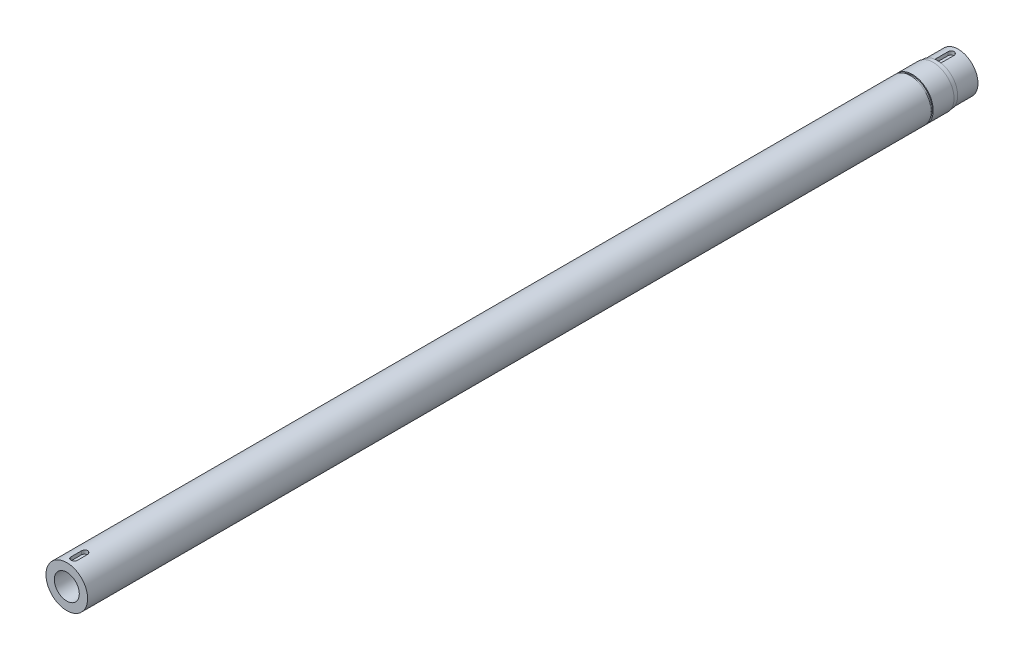
from build123d import *

# Parameters (mm, degrees)
SKETCH1_R           = 9.5
SKETCH1_R_2         = 6
BOSS_EXTRUDE1_DEPTH = 10
CUT_EXTRUDE1_DEPTH  = 1.8
CUT_EXTRUDE2_START  = 1.8
CUT_EXTRUDE2_DEPTH  = 1.8
SKETCH4_R           = 9.75
SKETCH4_R_2         = 6
BOSS_EXTRUDE2_DEPTH = 2
SKETCH5_R           = 10
BOSS_EXTRUDE3_DEPTH = 10
SKETCH6_R           = 6
CUT_EXTRUDE3_DEPTH  = 27.153393745
SKETCH7_R           = 9.5
SKETCH7_R_2         = 6
BOSS_EXTRUDE4_DEPTH = 1
SKETCH8_R           = 10
SKETCH8_R_2         = 6
BOSS_EXTRUDE5_DEPTH = 6
SKETCH9_R           = 10
SKETCH9_R_2         = 6
BOSS_EXTRUDE6_DEPTH = 150
SKETCH10_R          = 10
SKETCH10_R_2        = 6
BOSS_EXTRUDE7_DEPTH = 223
SKETCH11_R          = 10
SKETCH11_R_2        = 6
BOSS_EXTRUDE8_DEPTH = 26
CUT_EXTRUDE4_DEPTH  = 1.8


with BuildPart() as part:
    # Sketch1 → Boss-Extrude1 (new body)
    with BuildSketch(Plane.XY):
        Circle(SKETCH1_R)
        Circle(SKETCH1_R_2, mode=Mode.SUBTRACT)
    extrude(amount=BOSS_EXTRUDE1_DEPTH)

    # Sketch2 → Cut-Extrude1 (cut)
    with BuildSketch(Plane(origin=(0, 9.5, 0), x_dir=(1, 0, 0), z_dir=(0, 1, 0))):
        with BuildLine():
            Line((1.5, -3.5), (1.5, -8.5))
            Line((1.5, -8.5), (1.5, -10))
            Line((1.5, -10), (-1.5, -10))
            Line((-1.5, -10), (-1.5, -8.5))
            Line((-1.5, -8.5), (-1.5, -3.5))
            ThreePointArc((-1.5, -3.5), (0, -2), (1.5, -3.5))
        make_face()
    extrude(amount=-CUT_EXTRUDE1_DEPTH, mode=Mode.SUBTRACT)

    # Sketch3 → Cut-Extrude2 (cut)
    with BuildSketch(Plane(origin=(0, -9.5, 0), x_dir=(1, 0, 0), z_dir=(0, 1, 0)).offset(CUT_EXTRUDE2_START)):
        with BuildLine():
            Line((1.5, -3.5), (1.5, -8.5))
            Line((1.5, -8.5), (1.5, -10.030894453))
            Line((1.5, -10.030894453), (-1.5, -10.030894453))
            Line((-1.5, -10.030894453), (-1.5, -8.5))
            Line((-1.5, -8.5), (-1.5, -3.5))
            ThreePointArc((-1.5, -3.5), (0, -2), (1.5, -3.5))
        make_face()
    extrude(amount=-CUT_EXTRUDE2_DEPTH, mode=Mode.SUBTRACT)

    # Sketch4 → Boss-Extrude2 (add)
    with BuildSketch(Plane.XY.offset(10)):
        Circle(SKETCH4_R)
        Circle(SKETCH4_R_2, mode=Mode.SUBTRACT)
    extrude(amount=BOSS_EXTRUDE2_DEPTH)

    # Sketch5 → Boss-Extrude3 (add)
    with BuildSketch(Plane.XY.offset(12)):
        Circle(SKETCH5_R)
    extrude(amount=BOSS_EXTRUDE3_DEPTH)

    # Sketch6 → Cut-Extrude3 (cut, through all)
    with BuildSketch(Plane.XY.offset(22)):
        Circle(SKETCH6_R)
    extrude(amount=-CUT_EXTRUDE3_DEPTH, mode=Mode.SUBTRACT)

    # Sketch7 → Boss-Extrude4 (add)
    with BuildSketch(Plane.XY.offset(22)):
        with Locations(Location((0, 0, 0), (0, 0, 260.915279713))):
            Circle(SKETCH7_R)
        Circle(SKETCH7_R_2, mode=Mode.SUBTRACT)
    extrude(amount=BOSS_EXTRUDE4_DEPTH)

    # Sketch8 → Boss-Extrude5 (add)
    with BuildSketch(Plane.XY.offset(23)):
        Circle(SKETCH8_R)
        Circle(SKETCH8_R_2, mode=Mode.SUBTRACT)
    extrude(amount=BOSS_EXTRUDE5_DEPTH)

    # Sketch9 → Boss-Extrude6 (add)
    with BuildSketch(Plane.XY.offset(29)):
        Circle(SKETCH9_R)
        Circle(SKETCH9_R_2, mode=Mode.SUBTRACT)
    extrude(amount=BOSS_EXTRUDE6_DEPTH)

    # Sketch10 → Boss-Extrude7 (add)
    with BuildSketch(Plane.XY.offset(179)):
        Circle(SKETCH10_R)
        Circle(SKETCH10_R_2, mode=Mode.SUBTRACT)
    extrude(amount=BOSS_EXTRUDE7_DEPTH)

    # Sketch11 → Boss-Extrude8 (add)
    with BuildSketch(Plane.XY.offset(402)):
        Circle(SKETCH11_R)
        Circle(SKETCH11_R_2, mode=Mode.SUBTRACT)
    extrude(amount=BOSS_EXTRUDE8_DEPTH)

    # Sketch12 → Cut-Extrude4 (cut)
    with BuildSketch(Plane(origin=(0, 10, 0), x_dir=(1, 0, 0), z_dir=(0, 1, 0))):
        with BuildLine():
            Line((1.5, -419.5), (1.5, -424.5))
            ThreePointArc((1.5, -424.5), (0, -426), (-1.5, -424.5))
            Line((-1.5, -424.5), (-1.5, -419.5))
            ThreePointArc((-1.5, -419.5), (0, -418), (1.5, -419.5))
        make_face()
    extrude(amount=-CUT_EXTRUDE4_DEPTH, mode=Mode.SUBTRACT)


solid = part.part
